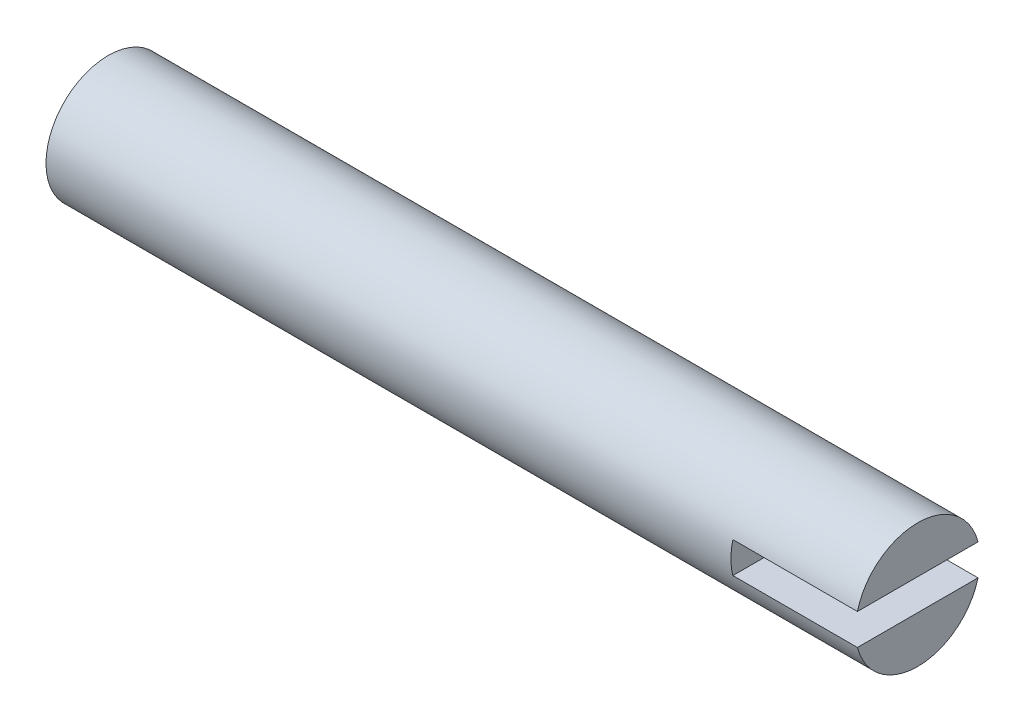
SolidWorks part; units mm, degrees
ref_plane "Front Plane" through (0, 0, 0) normal (0, 0, 1) x (1, 0, 0)
ref_plane "Top Plane" through (0, 0, 0) normal (0, 1, 0) x (1, 0, 0)
ref_plane "Right Plane" through (0, 0, 0) normal (1, 0, 0) x (0, 0, -1)
other "Configuration Table"
sketch "Sketch1" plane through (0, 0, 0) normal (1, 0, 0) x (0, 0, -1)
  circle A0 centre (0, 0) radius 1
  dimension "D1" = 2
extrude "Boss-Extrude1" add sketch "Sketch1" along normal blind 13
sketch "Sketch2" plane through (13, 0, 0) normal (1, 0, 0) x (0, 0, -1)
  line L1 (-1.2784, -0.25) -> (1.2784, -0.25)
  line L2 (-1.2784, -0.25) -> (-1.2784, 0.25)
  line L3 (-1.2784, 0.25) -> (1.2784, 0.25)
  line L4 (1.2784, -0.25) -> (1.2784, 0.25)
  line L5 (-1.2784, -0.25) -> (1.2784, 0.25) construction
  line L6 (-1.2784, 0.25) -> (1.2784, -0.25) construction
  point P0 (0, 0)
  dimension "D1" = 0.5
extrude "Cut-Extrude1" cut sketch "Sketch2" against normal blind 2
